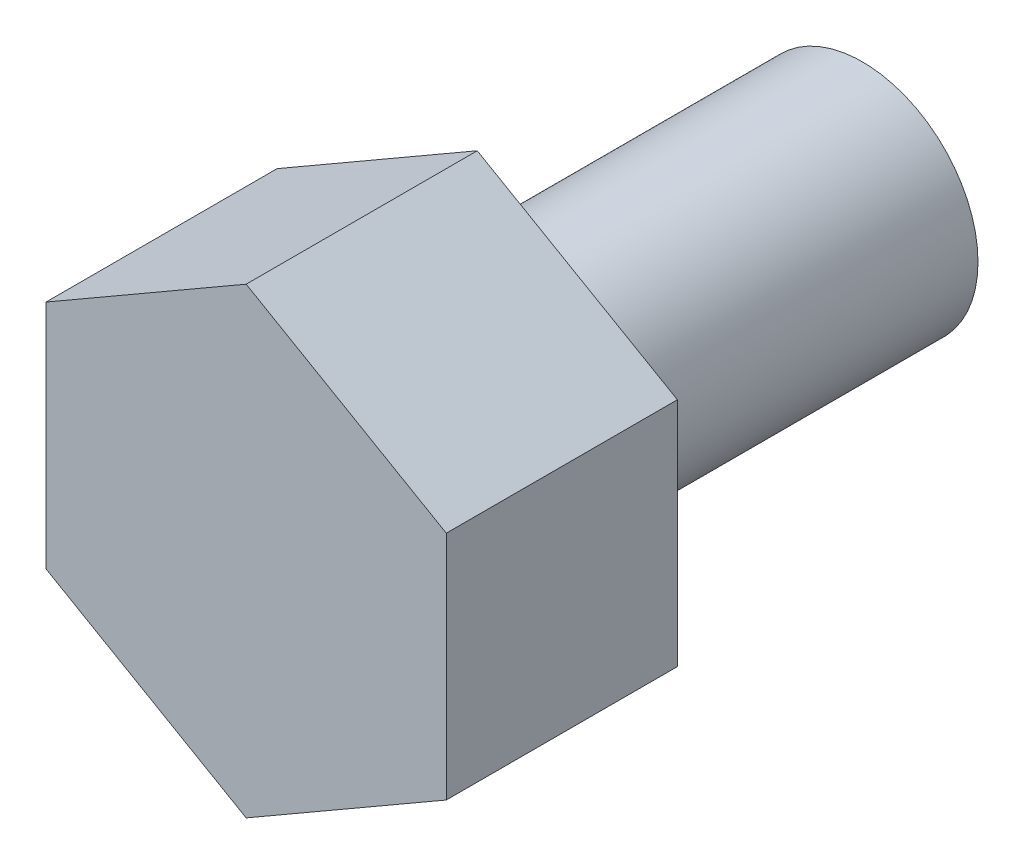
SolidWorks part; units mm, degrees
ref_plane "Front Plane" through (0, 0, 0) normal (0, 0, 1) x (1, 0, 0)
ref_plane "Top Plane" through (0, 0, 0) normal (0, 1, 0) x (1, 0, 0)
ref_plane "Right Plane" through (0, 0, 0) normal (1, 0, 0) x (0, 0, -1)
sketch "Sketch1" plane through (0, 0, 0) normal (0, 0, 1) x (1, 0, 0)
  circle A0 centre (0, 0) radius 3
  dimension "D1" = 6
extrude "Boss-Extrude1" add sketch "Sketch1" along normal blind 10
sketch "Sketch2" plane through (0, 0, 10) normal (0, 0, 1) x (1, 0, 0)
  line L1 (-5.1962, -3) -> (0, -6)
  line L2 (0, -6) -> (5.1962, -3)
  line L3 (5.1962, -3) -> (5.1962, 3)
  line L4 (5.1962, 3) -> (0, 6)
  line L5 (0, 6) -> (-5.1962, 3)
  line L6 (-5.1962, 3) -> (-5.1962, -3)
  circle A0 centre (0, 0) radius 5.1962 construction
  dimension "D1" = 12
extrude "Boss-Extrude2" add sketch "Sketch2" along normal blind 6
